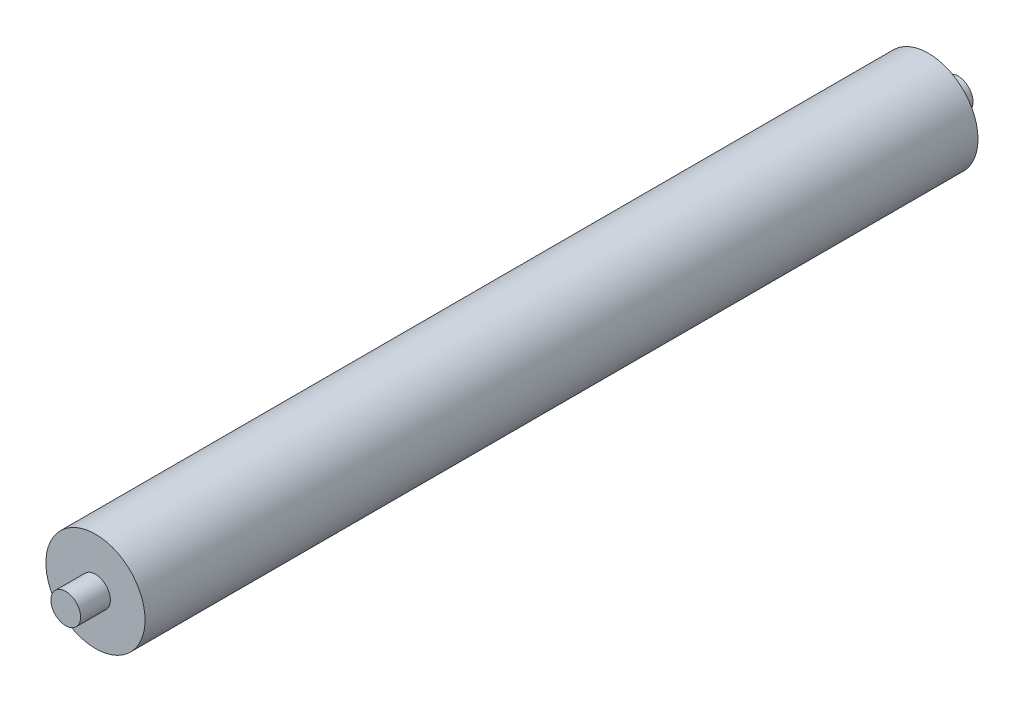
SolidWorks part; units mm, degrees
ref_plane "前视基准面" through (0, 0, 0) normal (0, 0, 1) x (1, 0, 0)
ref_plane "上视基准面" through (0, 0, 0) normal (0, 1, 0) x (1, 0, 0)
ref_plane "右视基准面" through (0, 0, 0) normal (1, 0, 0) x (0, 0, -1)
sketch "草图1" plane through (0, 0, 0) normal (0, 0, 1) x (1, 0, 0)
  circle A0 centre (0, 0) radius 25
  dimension "D1" = 50
extrude "凸台-拉伸1" add sketch "草图1" along normal blind 420
sketch "草图2" plane through (0, 0, 420) normal (0, 0, 1) x (1, 0, 0)
  circle A0 centre (0, 0) radius 7.5
  dimension "D1" = 15
extrude "凸台-拉伸2" add sketch "草图2" along normal blind 15
sketch "草图3" plane through (0, 0, 0) normal (0, 0, -1) x (-1, 0, 0)
  circle A0 centre (0, 0) radius 7.5
  dimension "D1" = 15
extrude "凸台-拉伸3" add sketch "草图3" along normal blind 15
